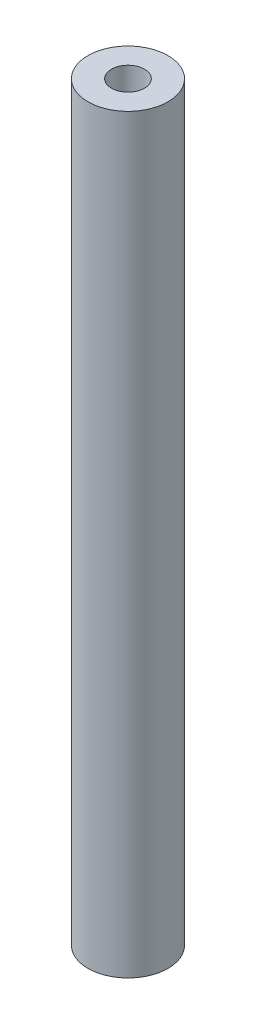
SolidWorks part; units mm, degrees
material "S45C"
ref_plane "前视基准面" through (0, 0, 0) normal (0, 0, 1) x (1, 0, 0)
ref_plane "上视基准面" through (0, 0, 0) normal (0, 1, 0) x (1, 0, 0)
ref_plane "右视基准面" through (0, 0, 0) normal (1, 0, 0) x (0, 0, -1)
sketch "草图1" plane through (0, 0, 0) normal (0, 1, 0) x (1, 0, 0)
  circle A0 centre (0, 0) radius 4
  dimension "D1" = 8
extrude "凸台-拉伸1" add sketch "草图1" along normal blind 75
hole_wizard "M4 螺纹孔1" positions "草图2" profile "草图3" tap size "M4" standard "GB"
sketch "草图2" plane through (0, 75, 0) normal (0, 1, 0) x (1, 0, 0)
  point P0 (0, 0)
sketch "草图3" plane through (0, 75, 0) normal (1, 0, 0) x (0, 0, 1)
  line L0 (0, 0) -> (0, 11.0914)
  line L1 (0, 11.0914) -> (1.65, 10.1)
  line L2 (1.65, 10.1) -> (1.65, 0)
  line L5 (1.65, 0) -> (0, 0)
  line L10 (0, 11.0914) -> (-1.65, 10.1) construction
  line L11 (0, -6.35) -> (0, 107.95) construction
  dimension "螺纹孔钻头直径" = 3.3
  dimension "螺纹孔钻头深度" = 10.1
  dimension "导头角度" = 118
cosmetic thread "孔螺蚊线1" parameters "D1"=8, "D2"=4
